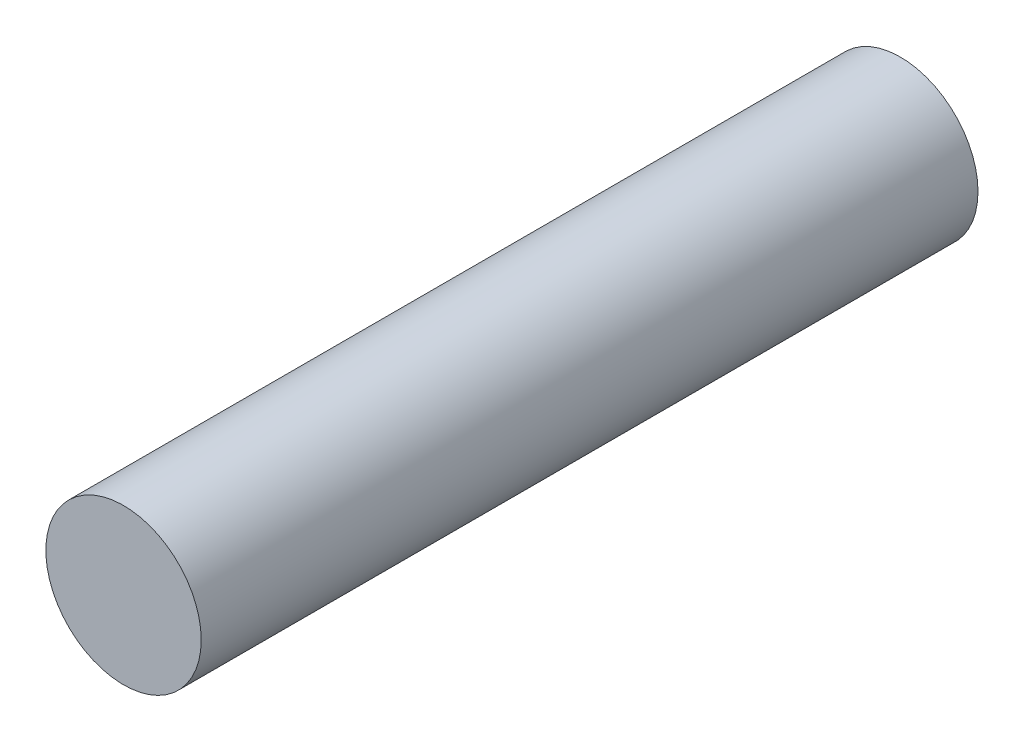
SolidWorks part; units mm, degrees
ref_plane "前视基准面" through (0, 0, 0) normal (0, 0, 1) x (1, 0, 0)
ref_plane "上视基准面" through (0, 0, 0) normal (0, 1, 0) x (1, 0, 0)
ref_plane "右视基准面" through (0, 0, 0) normal (1, 0, 0) x (0, 0, -1)
other "Configuration Table"
sketch "草图1" plane through (0, 0, 0) normal (0, 0, 1) x (1, 0, 0)
  circle A0 centre (0, 0) radius 6
  point P0 (0, 0)
  dimension "D1" = 12
extrude "凸台-拉伸1" add sketch "草图1" against normal mid plane 60
